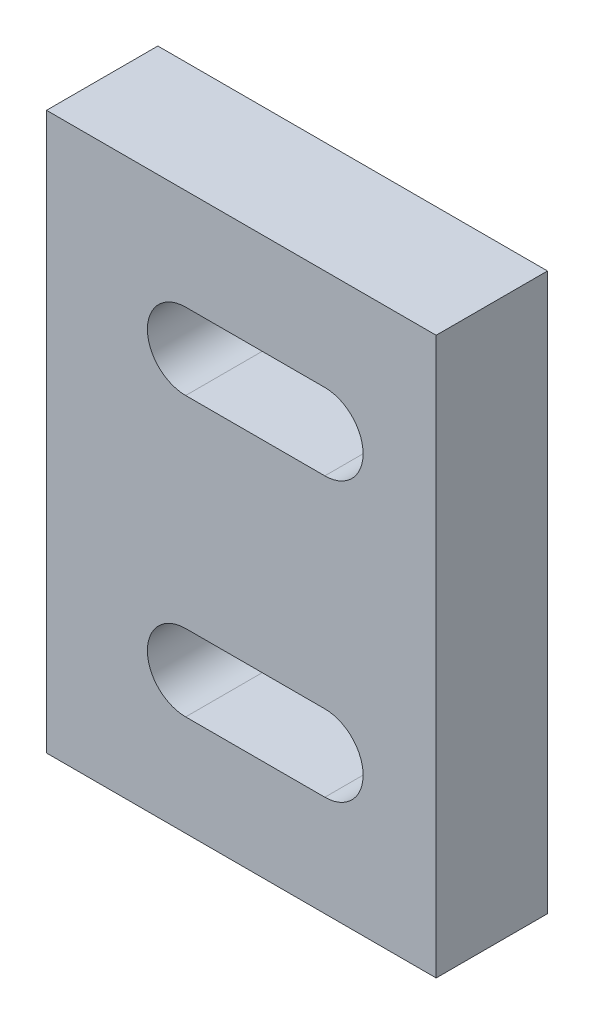
from build123d import *

# Parameters (mm, degrees)
SKETCH_1_W               = 56
SKETCH_1_H               = 80
EXTRUDE_1_DEPTH          = 16
CUT_EXTRUDE_1_DEPTH      = 52.380930315
CUT_EXTRUDE_1_DEPTH_BACK = 52.380930315


with BuildPart() as part:
    # 草图1 → 凸台-拉伸1 (new body)
    with BuildSketch(Plane.XY):
        Rectangle(SKETCH_1_W, SKETCH_1_H)
    extrude(amount=EXTRUDE_1_DEPTH)

    # 草图2 → 切除-拉伸1 (cut, two sides: drawn at the far end of the back side and taken through both)
    with BuildSketch(Plane(origin=(0, 0, 0), x_dir=(-1, 0, 0), z_dir=(0, 0, -1)).offset(-CUT_EXTRUDE_1_DEPTH_BACK)):
        with BuildLine():
            Line((-12, 25.5), (8, 25.5))
            ThreePointArc((8, 25.5), (13.5, 20), (8, 14.5))
            Line((8, 14.5), (-12, 14.5))
            ThreePointArc((-12, 14.5), (-17.5, 20), (-12, 25.5))
        make_face()
        with BuildLine():
            Line((-12, -25.5), (8, -25.5))
            ThreePointArc((8, -25.5), (13.5, -20), (8, -14.5))
            Line((8, -14.5), (-12, -14.5))
            ThreePointArc((-12, -14.5), (-17.5, -20), (-12, -25.5))
        make_face()
    extrude(amount=CUT_EXTRUDE_1_DEPTH + CUT_EXTRUDE_1_DEPTH_BACK, mode=Mode.SUBTRACT)


solid = part.part
